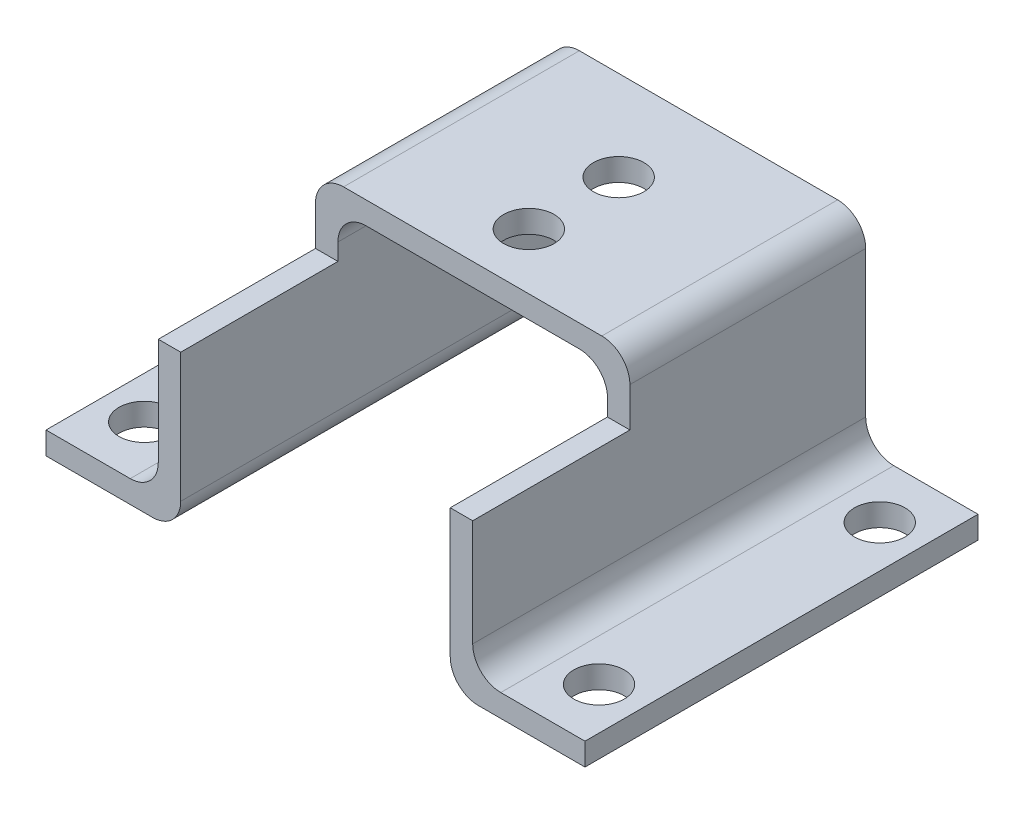
SolidWorks part; units mm, degrees
ref_plane "Front Plane" through (0, 0, 0) normal (0, 0, 1) x (1, 0, 0)
ref_plane "Top Plane" through (0, 0, 0) normal (0, 1, 0) x (1, 0, 0)
ref_plane "Right Plane" through (0, 0, 0) normal (1, 0, 0) x (0, 0, -1)
other "Configuration Table"
sketch "Sketch1" plane through (0, 0, 0) normal (0, 0, 1) x (1, 0, 0)
  line L0 (-24, 0) -> (-14.5, 0)
  line L1 (-12, 2.5) -> (-12, 15.5)
  line L2 (-9.5, 18) -> (9.5, 18)
  line L3 (12, 15.5) -> (12, 2.5)
  line L4 (14.5, 0) -> (24, 0)
  line L5 (-24, 2) -> (-16.5, 2)
  line L6 (-14, 4.5) -> (-14, 17.5)
  line L7 (-11.5, 20) -> (11.5, 20)
  line L8 (14, 17.5) -> (14, 4.5)
  line L9 (16.5, 2) -> (24, 2)
  line L10 (-24, 2) -> (-24, 0)
  line L11 (24, 2) -> (24, 0)
  line L12 (0, 20) -> (0, -20) construction
  line L13 (-14, 2) -> (-14, 20) construction
  line L14 (-14, 20) -> (14, 20) construction
  line L15 (14, 20) -> (14, 2) construction
  line L16 (-24, 2) -> (-14, 2) construction
  line L17 (14, 2) -> (24, 2) construction
  line L18 (12, 18) -> (12, 0) construction
  line L19 (12, 0) -> (24, 0) construction
  line L20 (-24, 0) -> (-12, 0) construction
  line L21 (-12, 0) -> (-12, 18) construction
  line L22 (-12, 18) -> (12, 18) construction
  arc A0 (-14, 17.5) -> (-11.5, 20) centre (-11.5, 17.5) cw
  arc A1 (14, 17.5) -> (11.5, 20) centre (11.5, 17.5) ccw
  arc A2 (-16.5, 2) -> (-14, 4.5) centre (-16.5, 4.5) ccw
  arc A3 (16.5, 2) -> (14, 4.5) centre (16.5, 4.5) cw
  arc A4 (12, 2.5) -> (14.5, 0) centre (14.5, 2.5) ccw
  arc A5 (-14.5, 0) -> (-12, 2.5) centre (-14.5, 2.5) ccw
  arc A6 (12, 15.5) -> (9.5, 18) centre (9.5, 15.5) ccw
  arc A7 (-12, 15.5) -> (-9.5, 18) centre (-9.5, 15.5) cw
  dimension "D5" = 2.5
  dimension "D6" = 2.5
  dimension "D1" = 24
  dimension "D3" = 48
  dimension "D4" = 20
  dimension "D2" = 2
extrude "Boss-Extrude1" add sketch "Sketch1" along normal blind 35
sketch "Sketch2" plane through (0, 0, 35) normal (0, 0, 1) x (1, 0, 0)
  line L0 (14.5, 0) -> (24, 0) construction
  line L1 (17.1964, 14) -> (-17.1964, 14)
  line L2 (17.1964, 14) -> (17.1964, 29.0376)
  line L3 (17.1964, 29.0376) -> (-17.1964, 29.0376)
  line L4 (-17.1964, 14) -> (-17.1964, 29.0376)
  line L5 (17.1964, 14) -> (-17.1964, 29.0376) construction
  line L6 (17.1964, 29.0376) -> (-17.1964, 14) construction
  point P0 (0, 21.5188)
  dimension "D1" = 14
extrude "Cut-Extrude1" cut sketch "Sketch2" against normal blind 14
sketch "Sketch3" plane through (0, 2, 0) normal (0, 1, 0) x (1, 0, 0)
  line L0 (0, 0) -> (0, 50000) construction
  line L1 (11.5, 0) -> (-11.5, 0) construction
  line L2 (-20.25, -35) -> (-20.25, 3.2471) construction
  line L3 (-16.5, -35) -> (-24, -35) construction
  line L4 (-16.5, 0) -> (-24, 0) construction
  circle A0 centre (-20.25, -5) radius 2.25
  circle A1 centre (-20.25, -30) radius 2.25
  circle A2 centre (20.25, -30) radius 2.25
  circle A3 centre (20.25, -5) radius 2.25
  circle A4 centre (0, -8) radius 2.25
  circle A5 centre (0, -16) radius 2.25
  point P4 (0, 0)
  dimension "D1" = 4.5
  dimension "D4" = 4.5
  dimension "D6" = 16
  dimension "D7" = 4.5
  dimension "D2" = 5
  dimension "D5" = 8
  dimension "D8" = 25
  dimension "D3" = 2
extrude "Cut-Extrude2" cut sketch "Sketch3" along normal mid plane 38
